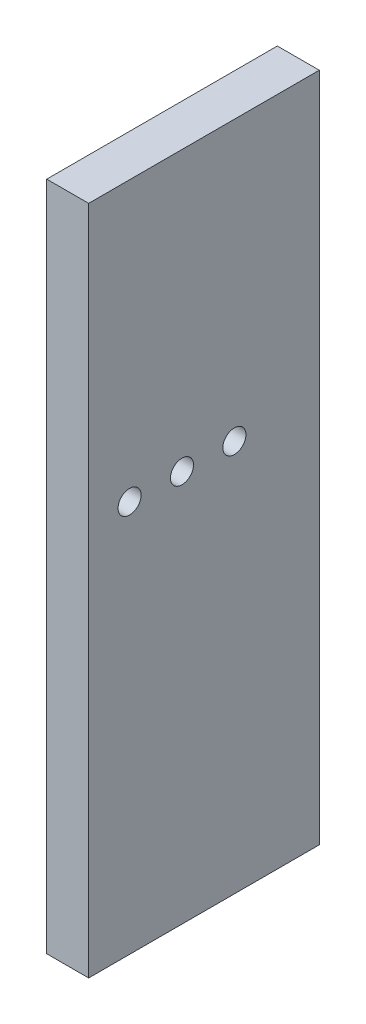
SolidWorks part; units mm, degrees
ref_plane "Front Plane" through (0, 0, 0) normal (0, 0, 1) x (1, 0, 0)
ref_plane "Top Plane" through (0, 0, 0) normal (0, 1, 0) x (1, 0, 0)
ref_plane "Right Plane" through (0, 0, 0) normal (1, 0, 0) x (0, 0, -1)
sketch "Sketch1" plane through (0, 0, 0) normal (0, 0, 1) x (1, 0, 0)
  line L1 (-120, 460) -> (-100, 460)
  line L2 (-120, 460) -> (-120, 140)
  line L3 (-120, 140) -> (-100, 140)
  line L4 (-100, 460) -> (-100, 140)
  dimension "D1" = 20
  dimension "D2" = 320
extrude "Boss-Extrude1" add sketch "Sketch1" along normal blind 110 contours L4 L3 L2 L1
hole_wizard "CBORE for M10 Hex Head Bolt1" positions "Sketch2" profile "Sketch3" counterbore size "M10" standard "GB"
sketch "Sketch2" plane through (-120, 0, 0) normal (-1, 0, 0) x (0, 0, 1)
  point P0 (40.49, 327)
  point P3 (65.49, 327)
  point P6 (90.49, 327)
sketch "Sketch3" plane through (-120, 327, 40.49) normal (0, 1, 0) x (0, 0, 1)
  line L0 (0, 0) -> (0, 25.5547)
  line L1 (0, 25.5547) -> (5.5, 22.25)
  line L2 (5.5, 22.25) -> (5.5, 10)
  line L3 (5.5, 10) -> (7.5, 10)
  line L4 (7.5, 10) -> (7.5, 0)
  line L5 (7.5, 0) -> (0, 0)
  line L10 (0, 25.5547) -> (-5.5, 22.25) construction
  line L11 (0, -6.35) -> (0, 107.95) construction
  dimension "孔直径" = 11
  dimension "孔深度" = 22.25
  dimension "柱形沉头孔直径" = 15
  dimension "柱形沉头孔深度" = 10
  dimension "导头角度" = 118
